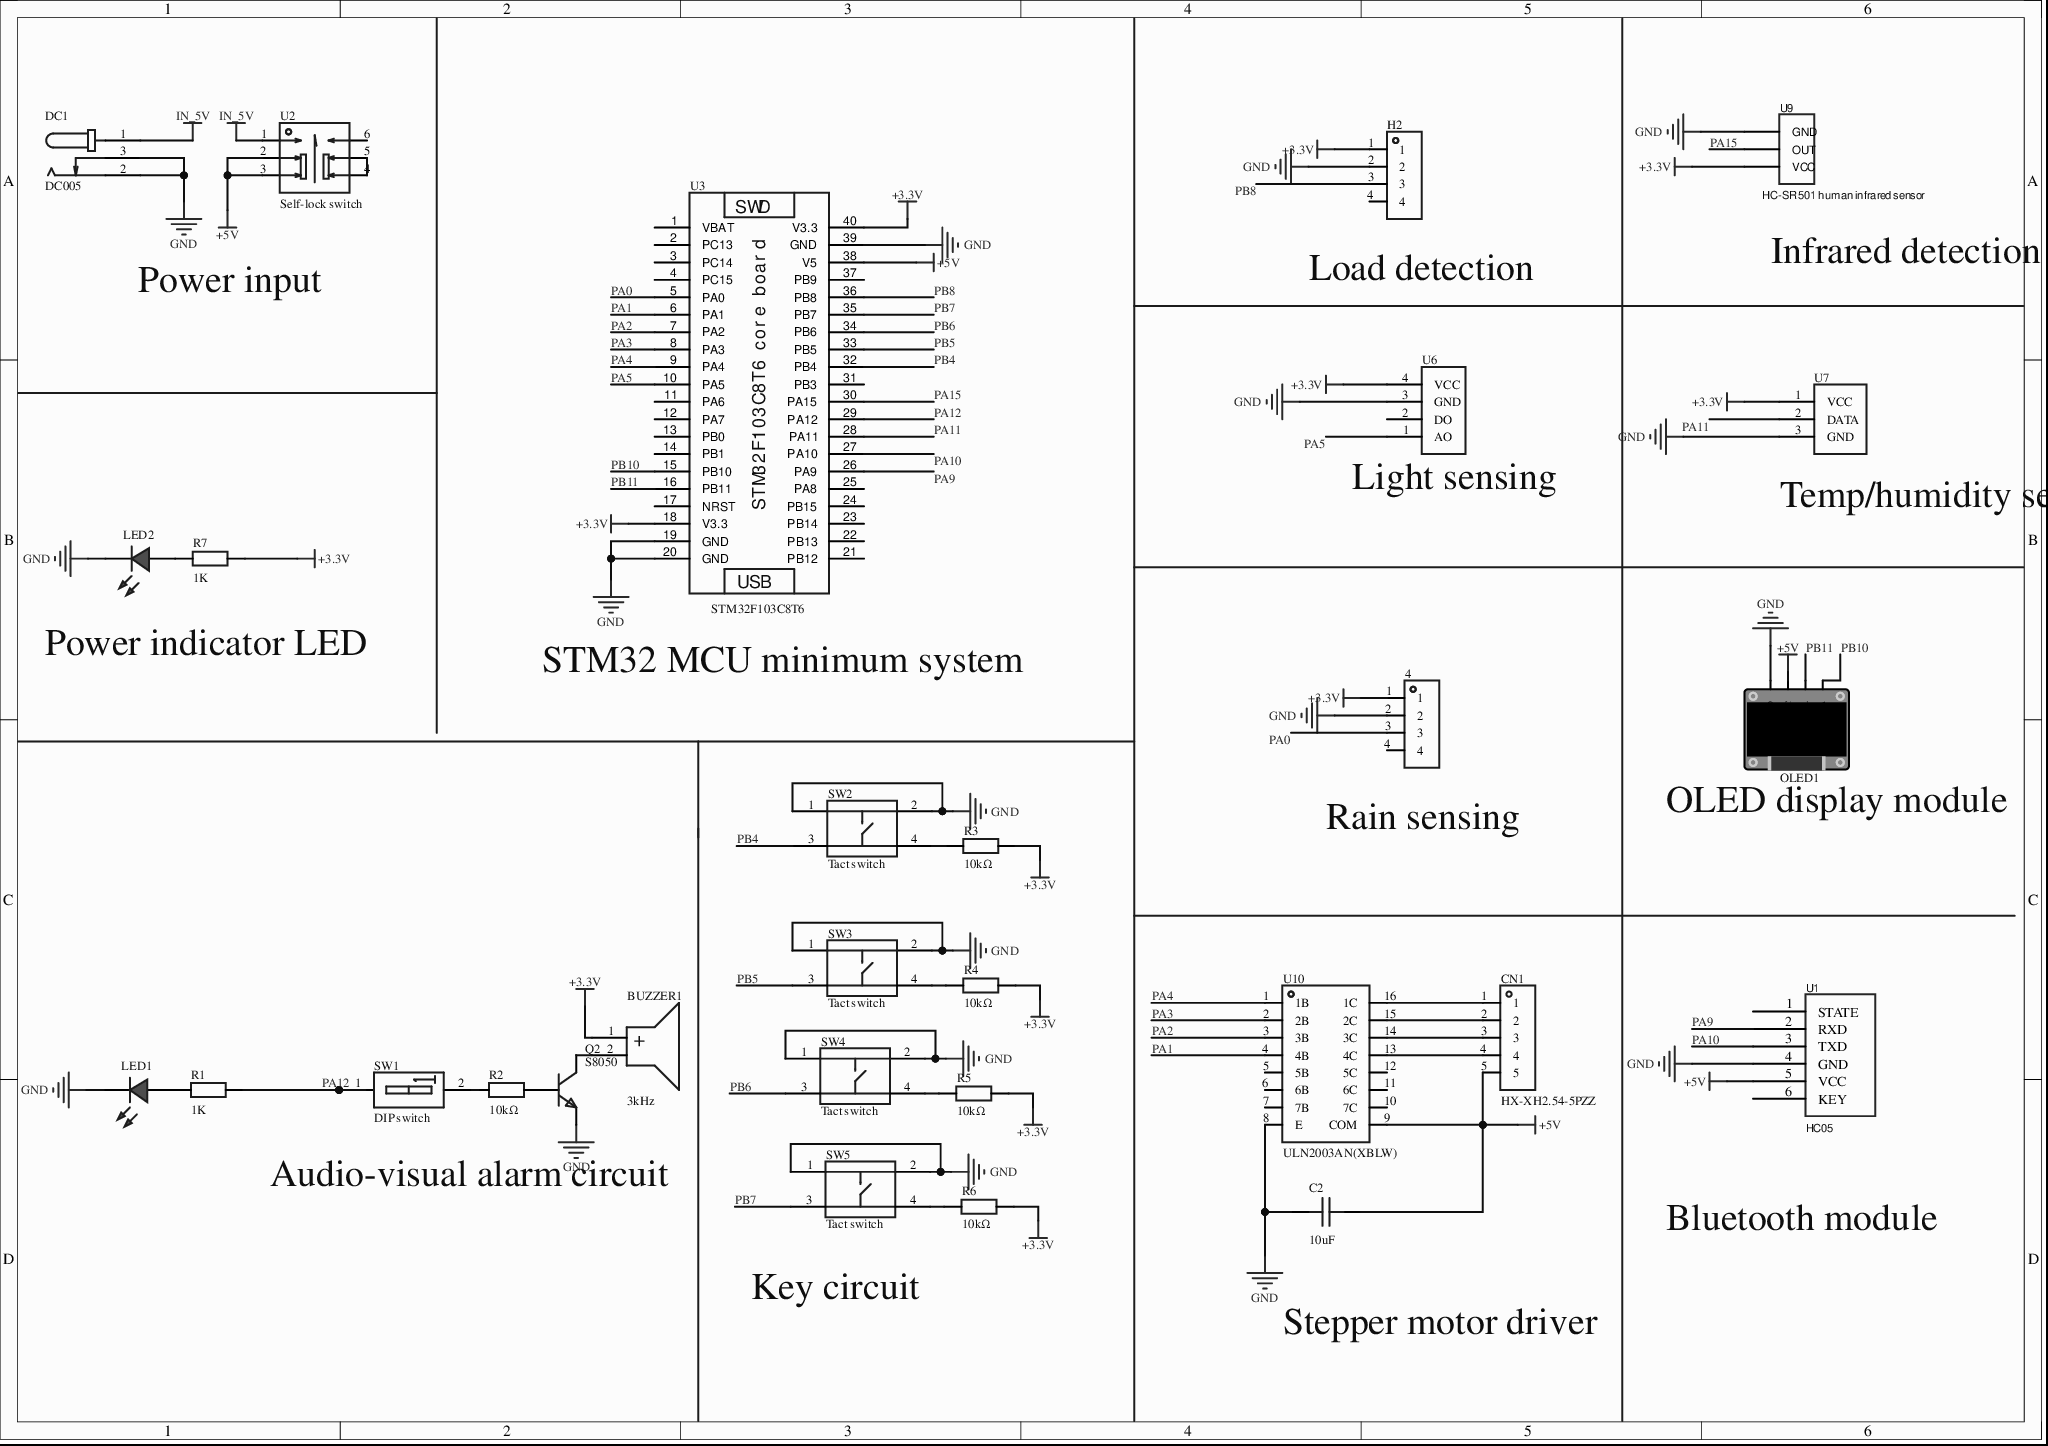
[diagram p0: MISC61241-3.schdoc]
# Altium project MISC61241-2.PrjPcb
1 sheet, 29 parts. Net scope: global (net labels, ports and power ports of the same name join across sheets).
Board file: MISC61241.pcbdoc

## Sheet MISC61241-3.schdoc
size 297 x 209 mm; Version: V1.0; @Project Name: MISC61241; @Update Date: 2026-04-29; @Create Date: 2026-04-29; @Board Name: MISC61241; @Create Time: 17:14:38; @Page Count: 1; @Page No: 1; @Schematic Name: MISC61241; @Update Time: 17:14:38; Size: A4

### Parts
4  (no value)  [HDR-TH_4P-P2.54-V-F]
BUZZER1  3kHz  [BUZZER]
C2  10uF  [CAP-TH_L10.0-W4.0-P7.50-D0.6-1]
CN1  HX-XH2.54-5PZZ  [CONN-TH_5P-P2.50_ZX-XH2.54-5PZZ]
DC1  DC005  [DC-IN-TH_DC005]
H2  (no value)  [HDR-TH_4P-P2.54-V-F]
LED1  (no value)  [LED-TH_5mm]
LED2  (no value)  [LED-TH_5mm]
OLED1  (no value)  [0.96OLED_4P]
Q2  S8050  [TO-92-3_L4.5-W3.5-P1.27-L]
R1  1K  [Res_1/4W]
R2  10kΩ  [Res_1/4W]
R3  10kΩ  [Res_1/4W]
R4  10kΩ  [Res_1/4W]
R5  10kΩ  [Res_1/4W]
R6  10kΩ  [Res_1/4W]
R7  1K  [Res_1/4W]
SW1  DIP switch  [SW-TH_DSWB01LHGET]
SW2  Tact switch  [KEY-TH_4P-L6.0-W6.0-P4.50-LS6.50]
SW3  Tact switch  [KEY-TH_4P-L6.0-W6.0-P4.50-LS6.50]
SW4  Tact switch  [KEY-TH_4P-L6.0-W6.0-P4.50-LS6.50]
SW5  Tact switch  [KEY-TH_4P-L6.0-W6.0-P4.50-LS6.50]
U1  HC05  [HC05]
U2  Self-lock switch  [SW-TH_6P-L5.8-W5.8-P2.00-LS4.5-TR]
U3  STM32F103C8T6  [STM32F103C8T6核心板]
U6  (no value)  [HDR-TH_4P-P2.54_342-40-104-00-592000]
U7  (no value)  [HDR-TH_3P-P2.54-V-M-B]
U9  HC-SR501 human infrared sensor  [大闸蟹-HC-SR501人体红外传感器]
U10  ULN2003AN(XBLW)  [PDIP-16_L19.3-W6.4-P2.54-LS7.9-BL]

### Nets
+3.3V: 4.1 BUZZER1.1(+) H2.1 R3.2 R4.2 R5.2 R6.2 R7.2 U3.18(V3.3) U3.40(V3.3) U6.4(VCC) U7.1(VCC) U9.3(VCC)
+5V: C2.2 CN1.5 OLED1.2(VCC) U1.5(VCC) U2.2 U2.3 U3.38(V5) U10.9(COM)
GND: 4.2 C2.1 DC1.2 DC1.3 H2.2 LED1.2(A) LED2.2(A) OLED1.1(GND) Q2.1(E) SW2.1 SW2.2 SW3.1 SW3.2 SW4.1 SW4.2 SW5.1 SW5.2 U1.4(GND) U3.19(GND) U3.20(GND) U3.39(GND) U6.3(GND) U7.3(GND) U9.1(GND) U10.8(E)
IN_5V: DC1.1 U2.1
PA0: 4.3 U3.5(PA0)
PA1: U3.6(PA1) U10.4(4B)
PA2: U3.7(PA2) U10.3(3B)
PA3: U3.8(PA3) U10.2(2B)
PA4: U3.9(PA4) U10.1(1B)
PA5: U3.10(PA5) U6.1(AO)
PA9: U1.2(RXD) U3.26(PA9)
PA10: U1.3(TXD) U3.27(PA10)
PA11: U3.28(PA11) U7.2(DATA)
PA12: R1.2 SW1.1(A1) U3.29(PA12)
PA15: U3.30(PA15) U9.2(OUT)
PB4: SW2.3 U3.32(PB4)
PB5: SW3.3 U3.33(PB5)
PB6: SW4.3 U3.34(PB6)
PB7: SW5.3 U3.35(PB7)
PB8: H2.3 U3.36(PB8)
PB10: OLED1.4(SDA) U3.15(PB10)
PB11: OLED1.3(SCL) U3.16(PB11)
NetBUZZER1_2: BUZZER1.2(-) Q2.3(C)
NetCN1_1: CN1.1 U10.16(1C)
NetCN1_2: CN1.2 U10.15(2C)
NetCN1_3: CN1.3 U10.14(3C)
NetCN1_4: CN1.4 U10.13(4C)
NetLED1_1: LED1.1(C) R1.1
NetLED2_1: LED2.1(C) R7.1
NetQ2_2: Q2.2(B) R2.2
NetR2_1: R2.1 SW1.2
NetR3_1: R3.1 SW2.4
NetR4_1: R4.1 SW3.4
NetR5_1: R5.1 SW4.4
NetR6_1: R6.1 SW5.4
NetU2_4: U2.4 U2.5

Not connected (* = marked no-connect by the designer): 4 4*; H2 4*; U1 1(STATE)* 6(KEY)*; U2 6*; U3 1(VBAT)* 2(PC13) 3(PC14) 4(PC15) 11(PA6) 12(PA7) 13(PB0) 14(PB1) 17(NRST) 21(PB12) 22(PB13) 23(PB14) 24(PB15) 25(PA8) 31(PB3) 37(PB9); U6 2(DO)*; U10 5(5B) 6(6B) 7(7B) 10(7C) 11(6C) 12(5C)

### Notes on the sheet
- Power input
- (near H2) Load detection
- (near U9) Infrared detection
- (near U6) Light sensing
- (near U7) Temp/humidity sensing
- Power indicator LED
- STM32 MCU minimum system
- (near 4) Rain sensing
- OLED display module
- Audio-visual alarm circuit
- Key circuit
- Bluetooth module
- Stepper motor driver

### Library data of the parts
4 H2 = HDR-F_2.54_1x4P: Symbol: 2.54-1*4P female; 3D Model: d187812051054f85879fcaa51a310d8e0819f05c4eef4c71ace90d822a990e87; 3D Model Transform: 419.6842,98.464,0,0,0,0,0,0,-118.11; ConvertToPcb: yes; Device: HDR-F_2.54_1x4P; Supplier Part: C2718488; Supplier Footprint: 插件; AddInBom: yes; FootprintName: HDR-TH_4P-P2.54-V-F; ModelName: HDR-TH_4P-P2.54-V-F
BUZZER1 = HNB09A03: Drive mode: active (built-in driver circuit); Construction type: electromagnetic; Frequency: 3kHz; Sound pressure (SPL): 85dB;; Manufacturer: 华能; AddInBom: yes; ModelId: 13273335caac486e928bafb4d9fdf12d0819f05c4eef4c71ace90d822a990e87; ModelName: BUZ-TH_D9.0-H5.5-P5.0; ModelTransform: 354.33,354.33,0,90,0,0,-0.005,0,-177.165; Voltage - Supply: 1.5V~4.5V; Current Consumption: 30mA; Symbol: HNB09A03; Device: HNB09A03; LCSC Part Name: 电磁式有源一体蜂鸣器HNB09A03; SupplierPart: C96102; ManufacturerPart: HNB09A03; Supplier Footprint: 插件,D=9mm; JLCPCB Part Class: Extended Part; Datasheet: example.com/datasheet/HNB09A03/97306.html; Supplier: LCSC; ConvertToPcb: yes; FootprintName: BUZZER; Driver Circuitry: Active (built-in driver circuit); Technology: Electromagnetic; Value: 3kHz; Sound Pressure Level(SPL): 85dB; Diameter(φD): 9mm; Length: -; Width: -; Height: 5.5mm; Operating Temperature: -20℃~+70℃
C2 = ECQU2A224ML: AddInBom: yes; ModelId: 58c4aaf12df94dde88df8b670b5e86d60819f05c4eef4c71ace90d822a990e87; ModelName: CAP-TH_L17.5-W7.8-H14.8-P15.0; ModelTransform: 688.975,307.086,0,0,0,0,-0.004,0,-137.795; Symbol: ECQU2A224ML; Device: ECQU2A224ML; LCSC Part Name: ECQU2A224ML; SupplierPart: C9900013261; ManufacturerPart: ECQU2A224ML; Supplier Footprint: CAP-TH_L17.5-W8.0-P15.00; JLCPCB Part Class: Extended Part; Supplier: LCSC; ConvertToPcb: yes; FootprintName: CAP-TH_L10.0-W4.0-P7.50-D0.6-1
CN1 = HX-XH2.54-5PZZ: Pin structure: 1x5P; Pitch: 2.54mm; Mounting: through-hole; Reference series: XH; Total pins: 5P; Rows: 1; Pins per row: 5; Row spacing: -; Rated current: 3A; Contact material: Brass; Contact plating: Tin; Operating temperature: -25℃~+85℃;; Manufacturer: hanxia(韩下); AddInBom: yes; ModelId: d05584c4f2494e6996f34343461d4ab00819f05c4eef4c71ace90d822a990e87; ModelTransform: 590.55,232.6767,0,0,0,0,0,14.528,-133.858; Number of PINs Per Row: 5; Voltage Rating: 250V; Plastic Material: PA66; Flame Retardant Rating: UL94V-0; Symbol: HX-XH2.54-5PZZ; Device: HX-XH2.54-5PZZ; LCSC Part Name: 1x5P 间距:2.5mm 直插 系列:XH; SupplierPart: C42391663; ManufacturerPart: HX-XH2.54-5PZZ; Supplier Footprint: 插件,P=2.5mm; JLCPCB Part Class: Extended Part; Datasheet: example.com/datasheet/HX-XH2.54-5PZZ/44326935.html; Supplier: LCSC; ConvertToPcb: yes; FootprintName: CONN-TH_5P-P2.50_ZX-XH2.54-5PZZ; ModelName: CONN-TH_5P-P2.50_ZX-XH2.54-5PZZ; Pins Structure: 1x5P; Mounting Type: Through-hole; Reference Series: XH; Number of Pins: 5P; Number of Rows: 1; Row Spacing: -; Current Rating: 3A; Contact Material: Brass; Contact Plating: Tin; Operating Temperature: -25℃~+85℃; Color: White
DC1 = DC005: Connector type: DC power jack; Mounting: right-angle; Contact inner diameter: 2mm; Contact outer diameter: 6.3mm; Rated current: 500mA; Rated voltage: 12V; Operating temperature: -30℃~+70℃;; Manufacturer: SHOU HAN(首韩); Symbol: DC005_C431533; AddInBom: yes; ModelId: f168fe383f964e0ea2af0127ff6ac7b40819f05c4eef4c71ace90d822a990e87; ModelTransform: 366.141,553.149,0,270,0,0,-141.734,88.583,-149.606; Device: DC005; LCSC Part Name: DC005-2.0 黑（铁）; SupplierPart: C431533; ManufacturerPart: DC005; Supplier Footprint: 插件; JLCPCB Part Class: Extended Part; Datasheet: example.com/datasheet/DC005/427890.html; Supplier: LCSC; ConvertToPcb: yes; FootprintName: DC-IN-TH_DC005; ModelName: DC-IN-TH_DC005; Connector Type: DC power jack; Mounting Type: Right-angle; Inside Contact Diameter: 2mm; Outside Contact Diameter: 6.3mm; Current Rating: 500mA; Voltage Rating (Max): 12V; Operating Temperature: -30℃~+70℃
LED1 LED2 = LED_TH-R_5mm: ConvertToPcb: yes; ModelId: fe9cea1bdf7642cd8d9a5077ed0e2b580819f05c4eef4c71ace90d822a990e87; ModelName: LED-TH_BD5.9-P2.54-RD_RED; ModelTransform: 222.16,238.98,581.81,180,0,0,-6,0,-220; Symbol: LED_TH-R; Device: LED_TH-R_5mm; AddInBom: yes; FootprintName: LED-TH_5mm; Supplier Footprint: 插件
OLED1 = 0.96OLED模块_4P: Symbol: 0.96OLED module_4P; ConvertToPcb: yes; ModelId: 79c000fdb68d45a296c2e9bedf4f90550819f05c4eef4c71ace90d822a990e87; ModelTransform: 1393.69792,1318.895,0,0,0,0,0,-560.079,-137.795; Device: 0.96OLED module_4P; AddInBom: yes; FootprintName: 0.96OLED_4P; Supplier Footprint: 插件; ModelName: 0.96OLED_4P
Q2 = S8050_C2931492: Transistor type: NPN; Collector current (Ic): 500mA; Collector-emitter breakdown voltage (Vceo): 25V; Power dissipation (Pd): 625mW; DC current gain (hFE): 160@50mA,1V;; Manufacturer: JSMSEMI(杰盛微); AddInBom: yes; ModelId: 45fa6cddef3743c6aacf8db740a3bc4c0819f05c4eef4c71ace90d822a990e87; ModelTransform: 177.165,137.795,0,0,0,0,0,29.528,-98.425; Transition frequency(fT): 150MHz; Current - Collector Cutoff: 100nA; Vce Saturation(VCE(sat)): 600mV@500mA,50mA; Emitter-Base Voltage(Vebo): 5V; Symbol: S8050_C2931492; Device: S8050_C2931492; LCSC Part Name: NPN 电流:500mA 电压:25V; SupplierPart: C2931492; ManufacturerPart: S8050; Supplier Footprint: TO-92; JLCPCB Part Class: Extended Part; Datasheet: example.com/datasheet/S8050/3272796.html; Supplier: LCSC; ConvertToPcb: yes; FootprintName: TO-92-3_L4.5-W3.5-P1.27-L; ModelName: TO-92-3_L4.5-W3.5-P1.27-L; type: NPN; Current - Collector(Ic): 500mA; Collector - Emitter Voltage VCEO: 25V; Pd - Power Dissipation: 625mW; DC Current Gain: 160@50mA,1V
R1 R7 = Res_AXIAL-1/4W: Symbol: Resistor; AddInBom: yes; ModelId: 463263665006444ab7a47bd11b0cf9560819f05c4eef4c71ace90d822a990e87; ModelName: RES-TH_BD2.4-L6.3-P10.30-D0.6; ModelTransform: 427.165,94.32816,0,0,0,0,0,0,-196.85; Value: 10kΩ; Device: Res_AXIAL-1/4W; Supplier Footprint: 轴向引线; ConvertToPcb: yes; FootprintName: Res_1/4W
R2-R6 = Res_AXIAL-1/4W: Symbol: Resistor; AddInBom: yes; ModelId: 463263665006444ab7a47bd11b0cf9560819f05c4eef4c71ace90d822a990e87; ModelName: RES-TH_BD2.4-L6.3-P10.30-D0.6; ModelTransform: 427.165,94.32816,0,0,0,0,0,0,-196.85; Device: Res_AXIAL-1/4W; Supplier Footprint: 轴向引线; ConvertToPcb: yes; FootprintName: Res_1/4W; Value: 10kΩ
SW1 = DSWB01LHGET: Type: slide, raised; Circuit structure: SPST; Number of positions: 1; Service life: -; Color: red;; Manufacturer: YE; AddInBom: yes; ModelId: 0f47cc4368c24d779ddaf17d8f9a8b630819f05c4eef4c71ace90d822a990e87; ModelName: SW-TH_2P-L4.1-W9.9-H5.4-P2.54; ModelTransform: 161.417,389.763,0,0,0,0,2.205,-1.024,-125.984; Number of Positions: 1 position; Symbol: DSWB01LHGET; Device: DSWB01LHGET; LCSC Part Name: 红色宽体1位顶拨插件; SupplierPart: C126888; ManufacturerPart: DSWB01LHGET; Supplier Footprint: 插件,9.9x4mm; JLCPCB Part Class: Extended Part; Datasheet: example.com/datasheet/DSWB01LHGET/138168.html; Supplier: LCSC; ConvertToPcb: yes; FootprintName: SW-TH_DSWB01LHGET; Type: Slide, raised; Circuit: SPST; Lead Pitch: -; Operating Life: -; Color: Red
SW2-SW5 = K2-1102DP-C4SW-04: Circuit structure: SPST; Button shape: round button; Actuating force: 2.5N; Mounting: through-hole; Switch length: 6mm; Switch width: 6mm; Switch height: 5mm; Contact current: 50mA; Rated voltage: 12V; With LED: -; Life: 10 ten-thousand cycles;; Manufacturer: 韩国韩荣; AddInBom: yes; ModelId: b38fea4b2e4e408486f1d54ff7bc5cc00819f05c4eef4c71ace90d822a990e87; ModelTransform: 307.086,236.22,0,0,0,0,0,0,-137.795; Symbol: K2-1102DP-C4SW-04; Device: K2-1102DP-C4SW-04; LCSC Part Name: 轻触按键开关6*6*5; SupplierPart: C110153; ManufacturerPart: K2-1102DP-C4SW-04; Supplier Footprint: 插件-4P,6x6mm; JLCPCB Part Class: Extended Part; Datasheet: example.com/datasheet/K2-1102DP-C4SW-04/111374.html; Supplier: LCSC; ConvertToPcb: yes; FootprintName: KEY-TH_4P-L6.0-W6.0-P4.50-LS6.50; ModelName: KEY-TH_4P-L6.0-W6.0-P4.50-LS6.50; Circuit: SPST; Actuator Style: Round button; Operating Force: 2.5N; Mounting Type: Through-hole; Length: 6mm; Width: 6mm; Switch Height: 5mm; Contact Current: 50mA; Voltage Rating: 12V; With Lamp: -; Life: 10 ten-thousand cycles; Operating Temperature: -25℃~+85℃
U2 = PB-22E85L: Self-lock/no-lock: self-lock;; Manufacturer: DEALON(德艺隆); AddInBom: yes; ModelId: 7e7b9e83d9ee4f02b9bae05764fb1b4b0819f05c4eef4c71ace90d822a990e87; ModelName: SW-TH_6P-L8.5-W8.5-P2.50-LS5.4-BL; ModelTransform: 334.645,346.456,0,90,0,0,5.907,0.004,-137.795; Symbol: PB-22E85L; Device: PB-22E85L; LCSC Part Name: PB-22E85L; SupplierPart: C5160826; ManufacturerPart: PB-22E85L; Supplier Footprint: 插件-6P,8.5x8.5mm; JLCPCB Part Class: Extended Part; Supplier: LCSC; ConvertToPcb: yes; FootprintName: SW-TH_6P-L5.8-W5.8-P2.00-LS4.5-TR; Self Lock / No Lock: Self-lock
U3 = STM32F103C8T6最小系统板: Manufacturer: 无; ManufacturerPart: STM32F103C8T6最小系统模块; Symbol: STM32F103C8T6 minimum system board; AddInBom: yes; tags: STM32; OriginFootprint: STM32F103C8T6 core board; Device: STM32F103C8T6 minimum system board; ConvertToPcb: yes; SupplierPart: C8734; JLCPCB Part Class: Basic Part; FootprintName: STM32F103C8T6 core board
U6 = 光敏电阻传感器: Symbol: Photoresistor sensor; AddInBom: yes; ModelId: 1c4389ca9c8443929a12830c080dd19b; Device: Photoresistor sensor; FootprintName: HDR-TH_4P-P2.54_342-40-104-00-592000; ConvertToPcb: yes; ModelName: HDR-TH_4P-P2.54_342-40-104-00-592000
U7 = dth11: AddInBom: yes; Symbol: dth11; Device: dth11; FootprintName: HDR-TH_3P-P2.54-V-M-B; ConvertToPcb: yes
U9 = HC-SR501人体红外传感器: Symbol: HC-SR501 human infrared sensor; Device: HC-SR501 human infrared sensor; FootprintName: HC-SR501 human infrared sensor
U10 = ULN2003AN(XBLW): Channels: seven; Collector-emitter breakdown voltage (Vceo): 50V; Collector current (Ic): 500mA;; Manufacturer: XBLW(芯伯乐); AddInBom: yes; ModelId: 7f4af0d2434d4264b3d074b3c8a801b50819f05c4eef4c71ace90d822a990e87; ModelTransform: 759.841,311.023,0,0,0,0,0,-0.001,-129.921; Voltage - Input(Max): 30V; Symbol: ULN2003AN(XBLW); Device: ULN2003AN(XBLW); LCSC Part Name: ULN2003AN; SupplierPart: C18723564; ManufacturerPart: ULN2003AN(XBLW); Supplier Footprint: DIP-16; JLCPCB Part Class: Extended Part; Datasheet: example.com/datasheet/ULN2003AN(XBLW)/19916691.html; Supplier: LCSC; ConvertToPcb: yes; FootprintName: PDIP-16_L19.3-W6.4-P2.54-LS7.9-BL; ModelName: PDIP-16_L19.3-W6.4-P2.54-LS7.9-BL; number of channels: seven; Collector - Emitter Voltage VCEO: 50V; Current - Collector(Ic): 500mA; Operating Temperature: -
U1 = HC05: Symbol: HC05; Device: HC05; FootprintName: HC05